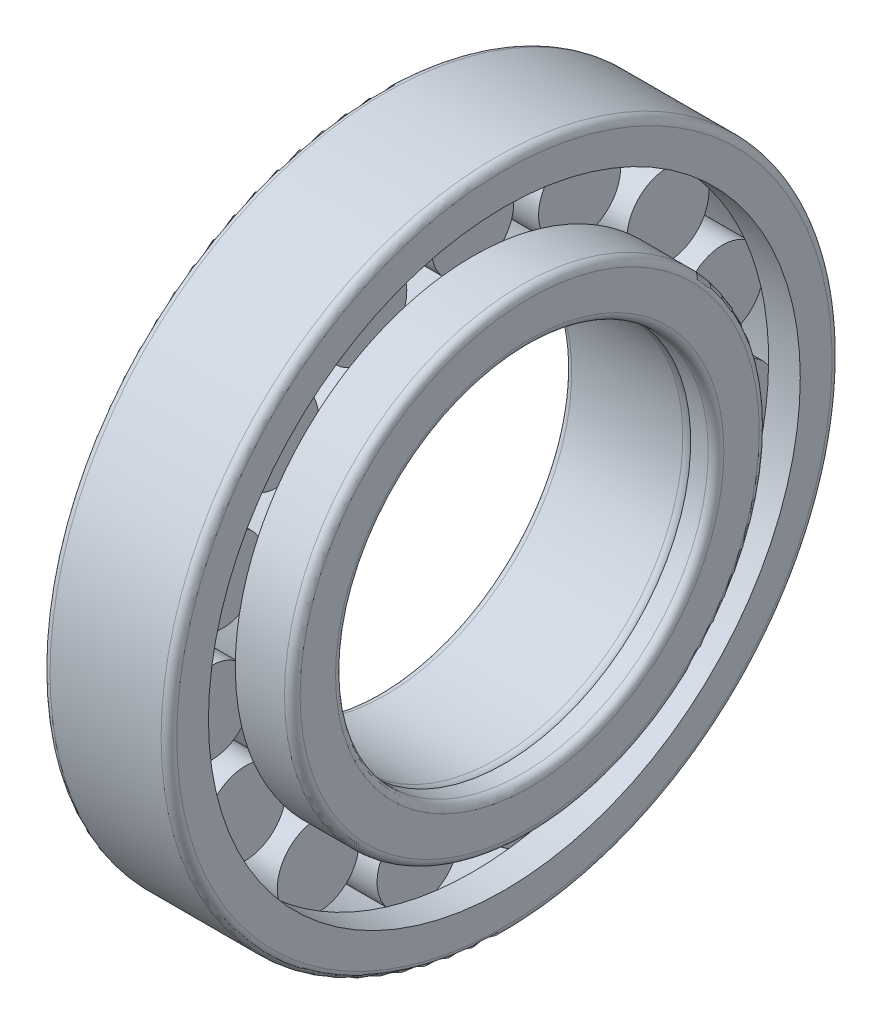
SolidWorks part; units mm, degrees
revolve "基体-旋转" add sketch "草图2" angle 360 about L0
sketch "草图2" plane through (0, 0, 0) normal (0, 0, 1) x (1, 0, 0)
  line L0 (-10.0801, 0) -> (21.9267, 0) construction
  line L1 (8.5, 59.5) -> (25.5, 59.5)
  line L2 (0, 63.7) -> (8.5, 63.7)
  line L3 (0, 63.7) -> (0, 52.1)
  line L4 (2.1, 50) -> (31.9, 50)
  line L5 (34, 57.2224) -> (34, 52.1)
  line L6 (8.5, 59.5) -> (8.5, 63.7)
  line L7 (34, 57.2224) -> (25.5, 59.5)
  arc A0 (31.9, 50) -> (34, 52.1) centre (31.9, 52.1) ccw
  arc A1 (0, 52.1) -> (2.1, 50) centre (2.1, 52.1) ccw
  point P13 (34, 50)
  point P16 (0, 50)
revolve "凸台-旋转1" add sketch "草图3" angle 360 about L2
sketch "草图3" plane through (0, 0, 0) normal (0, 0, 1) x (1, 0, 0)
  line L1 (25.5, 59.5) -> (25.5, -59.5) construction
  line L2 (-1.6039, 70.5) -> (13.5036, 70.5) construction
  line L4 (8.5, 70.5) -> (25.5, 70.5)
  line L5 (8.5, 70.5) -> (8.5, 59.4999)
  line L6 (8.5, 59.4999) -> (25.5, 59.4999)
  line L7 (25.5, 70.5) -> (25.5, 59.4999)
  line L8 (8.5, -63.7) -> (8.5, 63.7) construction
  dimension "D1" = 70.5
  dimension "D2" = 11.0001
revolve "凸台-旋转2" add sketch "草图4" angle 360 about L0
sketch "草图4" plane through (0, 0, 0) normal (0, 0, 1) x (1, 0, 0)
  line L0 (0, 0) -> (17.8006, 0) construction
  line L1 (-10.0801, 0) -> (21.9267, 0) construction
  line L2 (25.5, 79.4) -> (34, 79.4)
  line L3 (2.1, 90) -> (31.9, 90)
  line L4 (0, 87.9) -> (0, 79.4)
  line L5 (0, 79.4) -> (8.5, 79.4)
  line L6 (34, 87.9) -> (34, 79.4)
  line L7 (8.5, 81.5) -> (25.5, 81.5)
  line L8 (8.5, 81.5) -> (8.5, 79.4)
  line L10 (25.5, 81.5) -> (25.5, 79.4)
  arc A0 (31.9, 90) -> (34, 87.9) centre (31.9, 87.9) cw
  arc A1 (2.1, 90) -> (0, 87.9) centre (2.1, 87.9) ccw
  point P15 (34, 90)
  point P18 (0, 90)
material "GCr4"
ref_plane "基准面1" through (0, 0, 0) normal (0, 0, 1) x (1, 0, 0)
ref_plane "基准面2" through (0, 0, 0) normal (0, 1, 0) x (1, 0, 0)
ref_plane "基准面3" through (0, 0, 0) normal (1, 0, 0) x (0, 0, -1)
sketch "尺寸草图" plane through (0, 0, 0) normal (0, 0, 1) x (1, 0, 0)
  line L0 (0, 0) -> (2.1, 0)
  line L1 (2.1, 0) -> (4.2, 0)
  line L2 (4.2, 0) -> (38.2, 0)
  line L3 (38.2, 0) -> (138.2, 0)
  line L4 (138.2, 0) -> (257.2, 0)
  line L5 (257.2, 0) -> (437.2, 0)
  line L6 (600.2, 0) -> (607, 0)
  line L7 (437.2, 0) -> (600.2, 0)
sketch "草图5" plane through (0, 0, 0) normal (0, 0, 1) x (1, 0, 0)
  line L0 (0, 0) -> (19.6659, 0) construction
  line L1 (-10.0801, 0) -> (21.9267, 0) construction
  line L2 (34, 57.2224) -> (34, 50)
  line L3 (34, -57.2224) -> (34, 57.2224) construction
  line L4 (34, -52.1) -> (34, 52.1) construction
  line L5 (34, 57.2224) -> (25.5, 59.5)
  line L6 (34, -79.4) -> (34, 79.4) construction
  line L7 (25.5, 59.5) -> (25.5, 63.7)
  line L8 (25.5, 63.7) -> (38.7, 63.7)
  line L9 (40.8, 61.6) -> (40.8, 52.1)
  line L10 (38.7, 50) -> (34, 50)
  arc A0 (38.7, 63.7) -> (40.8, 61.6) centre (38.7, 61.6) cw
  arc A1 (38.7, 50) -> (40.8, 52.1) centre (38.7, 52.1) ccw
revolve "凸台-旋转3" add sketch "草图5" angle 360 about L0
pattern_circular "阵列(圆周)1" count 15 over 360 about axis through (0, 0, 0) along (1, 0, 0) of "凸台-旋转1"
equation "\"DD@草图2\" = \"内径@尺寸草图\""
equation "\"FW@草图2\" = \"参考FW@尺寸草图\""
equation "\"D1@草图2\" = \"倒角小@尺寸草图\""
equation "\"EW@草图4\" = \"参考EW@尺寸草图\""
equation "\"B@草图4\" = \"宽度@尺寸草图\""
equation "\"D@草图4\" = \"外径@尺寸草图\""
equation "\"D2@草图4\" = \"倒角大@尺寸草图\""
equation "\"架宽度@尺寸草图\" = 0.20*\"宽度@尺寸草图\""
equation "\"D5@草图5\" = \"架宽度@尺寸草图\""
equation "\"D4@草图2\" = \"FW@草图2\" + 4 *\"D1@草图2\""
equation "\"D2@草图2\" = \"B@草图4\""
equation "\"滚珠位置@草图2\" = \"D2@草图2\"/4"
equation "\"D3@草图4\" = \"D2@草图4\""
equation "\"D1@草图3\" =  ( \"EW@草图4\" - \"FW@草图2\" )  / 4 + \"FW@草图2\" / 2"
equation "\"D2@草图3\" =  0.25*( \"EW@草图4\" - \"FW@草图2\" ) +0.0001"
equation "\"D1@阵列(圆周)1\" =0.75* \"D1@草图3\" * 3.14 / \"D2@草图3\""
equation "\"D1@草图5\" = \"D1@草图2\""
equation "\"D4@草图5\" = \"D4@草图2\""
equation "\"D2@草图5\" = \"DD@草图2\""
